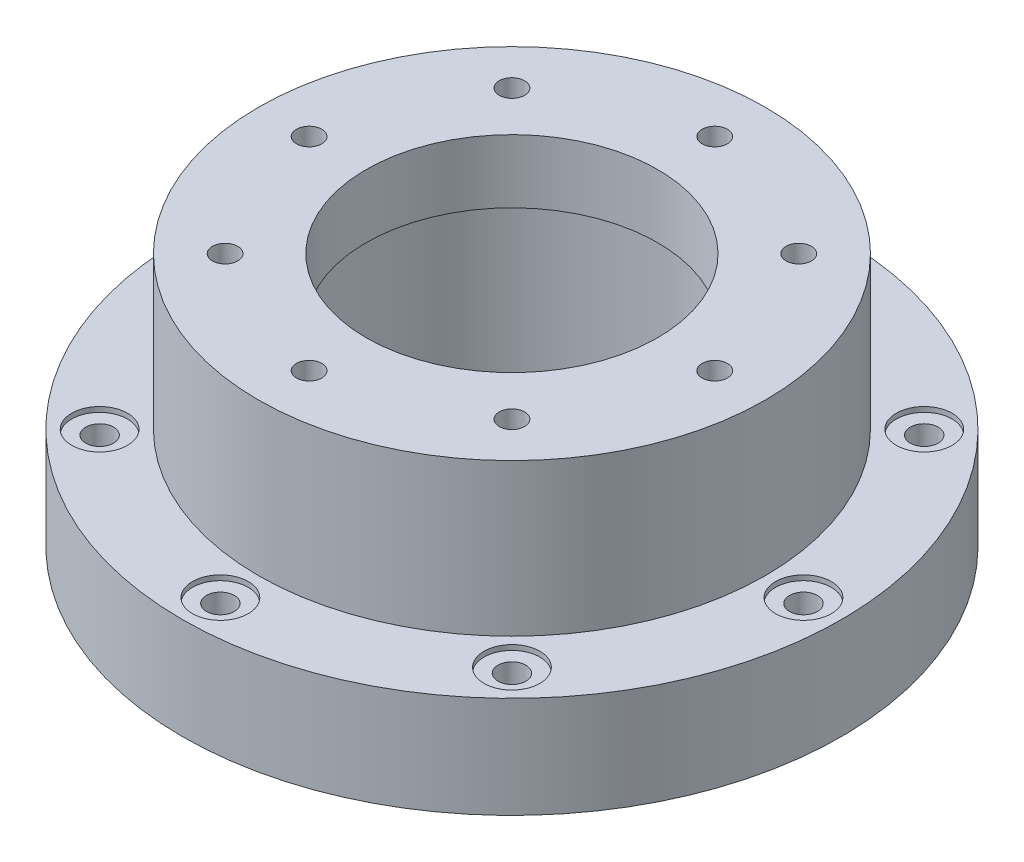
SolidWorks part; units mm, degrees
ref_plane "前视基准面" through (0, 0, 0) normal (0, 0, 1) x (1, 0, 0)
ref_plane "上视基准面" through (0, 0, 0) normal (0, 1, 0) x (1, 0, 0)
ref_plane "右视基准面" through (0, 0, 0) normal (1, 0, 0) x (0, 0, -1)
sketch "草图1" plane through (0, 0, 0) normal (0, 0, 1) x (1, 0, 0)
  line L0 (0, 133.6875) -> (0, -146.9125) construction
  line L1 (65, 35) -> (57.5, 35)
  line L2 (57.5, 35) -> (57.5, 60)
  line L3 (57.5, 60) -> (100, 60)
  line L4 (100, 60) -> (100, 0)
  line L5 (100, 0) -> (130, 0)
  line L6 (130, 0) -> (130, -40)
  line L7 (130, -40) -> (87.5, -40)
  line L8 (77.5, -50) -> (77.5, -65)
  line L9 (77.5, -65) -> (65, -65)
  line L10 (65, -65) -> (65, 35)
  arc A0 (77.5, -50) -> (87.5, -40) centre (87.5, -50) cw
  point P15 (77.5, -40)
  dimension "D10" = 10
  dimension "D1" = 57.5
  dimension "D2" = 42.5
  dimension "D3" = 7.5
  dimension "D4" = 30
  dimension "D5" = 52.5
  dimension "D6" = 25
  dimension "D7" = 60
  dimension "D8" = 40
  dimension "D9" = 25
revolve "旋转1" add sketch "草图1" angle 360 about L0
sketch "草图2" plane through (0, 0, 0) normal (0, 1, 0) x (1, 0, 0)
  circle A0 centre (115, 0) radius 11
  circle A1 centre (81.3173, -81.3173) radius 11
  circle A2 centre (0, -115) radius 11
  circle A3 centre (-81.3173, -81.3173) radius 11
  circle A4 centre (-115, 0) radius 11
  circle A5 centre (-81.3173, 81.3173) radius 11
  circle A6 centre (0, 115) radius 11
  circle A7 centre (81.3173, 81.3173) radius 11
  point P19 (0, 0)
  dimension "D1" = 22
  dimension "D2" = 115
  dimension "D3" = 8
extrude "切除-拉伸1" cut sketch "草图2" against normal blind 2
sketch "草图3" plane through (0, -2, 0) normal (0, 1, 0) x (1, 0, 0)
  circle A0 centre (81.3173, 81.3173) radius 5.5
  circle A1 centre (115, 0) radius 5.5
  circle A2 centre (81.3173, -81.3173) radius 5.5
  circle A3 centre (0, -115) radius 5.5
  circle A4 centre (-81.3173, -81.3173) radius 5.5
  circle A5 centre (-115, 0) radius 5.5
  circle A6 centre (-81.3173, 81.3173) radius 5.5
  circle A7 centre (0, 115) radius 5.5
  point P19 (0, 0)
  dimension "D1" = 11
  dimension "D2" = 8
extrude "切除-拉伸2" cut sketch "草图3" against normal up to next
sketch "草图4" plane through (0, 60, 0) normal (0, 1, 0) x (1, 0, 0)
  circle A0 centre (80, 0) radius 5
  circle A1 centre (56.5685, -56.5685) radius 5
  circle A2 centre (0, -80) radius 5
  circle A3 centre (-56.5685, -56.5685) radius 5
  circle A4 centre (-80, 0) radius 5
  circle A5 centre (-56.5685, 56.5685) radius 5
  circle A6 centre (0, 80) radius 5
  circle A7 centre (56.5685, 56.5685) radius 5
  point P19 (0, 0)
  dimension "D1" = 10
  dimension "D2" = 80
  dimension "D3" = 8
extrude "切除-拉伸3" cut sketch "草图4" against normal blind 46
